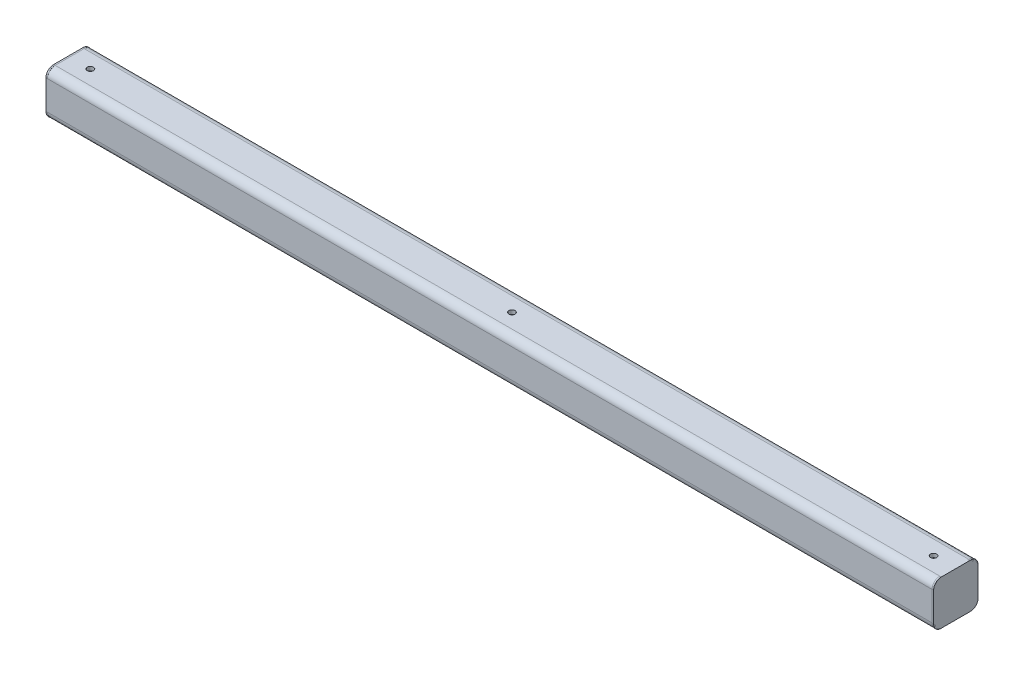
from build123d import *

# Parameters (mm, degrees)
MEMBER_1_DEPTH              = 600
EXTRUDE_1_DEPTH             = 1
EXTRUDE_2_DEPTH             = 1
SKETCH_5_W                  = 2.1
SKETCH_5_H                  = 30
HOLE_WIZARD_M5_1_AT_2_COUNT = 2
HOLE_WIZARD_M5_1_AT_2_PITCH = 285
HOLE_WIZARD_M5_1_AT_3_COUNT = 2
HOLE_WIZARD_M5_1_AT_3_PITCH = 570


with BuildPart() as part:
    # Sketch1 → Member 1 (new body)
    with BuildSketch(Plane(origin=(0, 0, 0), x_dir=(0, 0, -1), z_dir=(1, 0, 0))):
        with BuildLine():
            Line((-9.8, -15), (9.8, -15))
            ThreePointArc((9.8, -15), (13.476955262, -13.476955262), (15, -9.8))
            Line((15, -9.8), (15, 9.8))
            ThreePointArc((15, 9.8), (13.476955262, 13.476955262), (9.8, 15))
            Line((9.8, 15), (-9.8, 15))
            ThreePointArc((-9.8, 15), (-13.476955262, 13.476955262), (-15, 9.8))
            Line((-15, 9.8), (-15, -9.8))
            ThreePointArc((-15, -9.8), (-13.476955262, -13.476955262), (-9.8, -15))
        make_face()
        with BuildLine():
            Line((-9.8, -12.4), (9.8, -12.4))
            ThreePointArc((9.8, -12.4), (11.638477631, -11.638477631), (12.4, -9.8))
            Line((12.4, -9.8), (12.4, 9.8))
            ThreePointArc((12.4, 9.8), (11.638477631, 11.638477631), (9.8, 12.4))
            Line((9.8, 12.4), (-9.8, 12.4))
            ThreePointArc((-9.8, 12.4), (-11.638477631, 11.638477631), (-12.4, 9.8))
            Line((-12.4, 9.8), (-12.4, -9.8))
            ThreePointArc((-12.4, -9.8), (-11.638477631, -11.638477631), (-9.8, -12.4))
        make_face(mode=Mode.SUBTRACT)
    extrude(amount=MEMBER_1_DEPTH)

    # 草图5 → M5 螺纹孔1 (revolve, cut)
    with BuildSketch(Plane(origin=(14.999999998, -15, 1e-09), x_dir=(0, 0, -1), z_dir=(1, 0, 0))):
        with Locations((1.05, 15)):
            Rectangle(SKETCH_5_W, SKETCH_5_H)
    hole_wizard_m5_1 = revolve(axis=Axis((14.999999998, -21.35, 1e-09), (0, 1, 0)), mode=Mode.SUBTRACT)

    # M5 螺纹孔1 at 2: M5 螺纹孔1 ×2
    with Locations(*[(i * HOLE_WIZARD_M5_1_AT_2_PITCH, 0, 0) for i in range(1, HOLE_WIZARD_M5_1_AT_2_COUNT)]):
        add(hole_wizard_m5_1, mode=Mode.SUBTRACT)

    # M5 螺纹孔1 at 3: M5 螺纹孔1 ×2
    with Locations(*[(i * HOLE_WIZARD_M5_1_AT_3_PITCH, 0, 0) for i in range(1, HOLE_WIZARD_M5_1_AT_3_COUNT)]):
        add(hole_wizard_m5_1, mode=Mode.SUBTRACT)


with BuildPart() as body_2:
    # 草图1 → 凸台-拉伸1 (new body)
    with BuildSketch(Plane.ZY):
        with BuildLine():
            Line((10, 15), (-10, 15))
            ThreePointArc((-10, 15), (-13.535533906, 13.535533906), (-15, 10))
            Line((-15, 10), (-15, -10))
            ThreePointArc((-15, -10), (-13.535533906, -13.535533906), (-10, -15))
            Line((-10, -15), (10, -15))
            ThreePointArc((10, -15), (13.535533906, -13.535533906), (15, -10))
            Line((15, -10), (15, 10))
            ThreePointArc((15, 10), (13.535533906, 13.535533906), (10, 15))
        make_face()
    extrude(amount=-EXTRUDE_1_DEPTH)


with BuildPart() as body_3:
    # 草图2 → 凸台-拉伸2 (new body)
    with BuildSketch(Plane(origin=(600, 0, 0), x_dir=(0, 0, -1), z_dir=(1, 0, 0))):
        with BuildLine():
            Line((10, 15), (-10, 15))
            ThreePointArc((-10, 15), (-13.535533906, 13.535533906), (-15, 10))
            Line((-15, 10), (-15, -10))
            ThreePointArc((-15, -10), (-13.535533906, -13.535533906), (-10, -15))
            Line((-10, -15), (10, -15))
            ThreePointArc((10, -15), (13.535533906, -13.535533906), (15, -10))
            Line((15, -10), (15, 10))
            ThreePointArc((15, 10), (13.535533906, 13.535533906), (10, 15))
        make_face()
    extrude(amount=-EXTRUDE_2_DEPTH)


solid = Compound([part.part, body_2.part, body_3.part])
